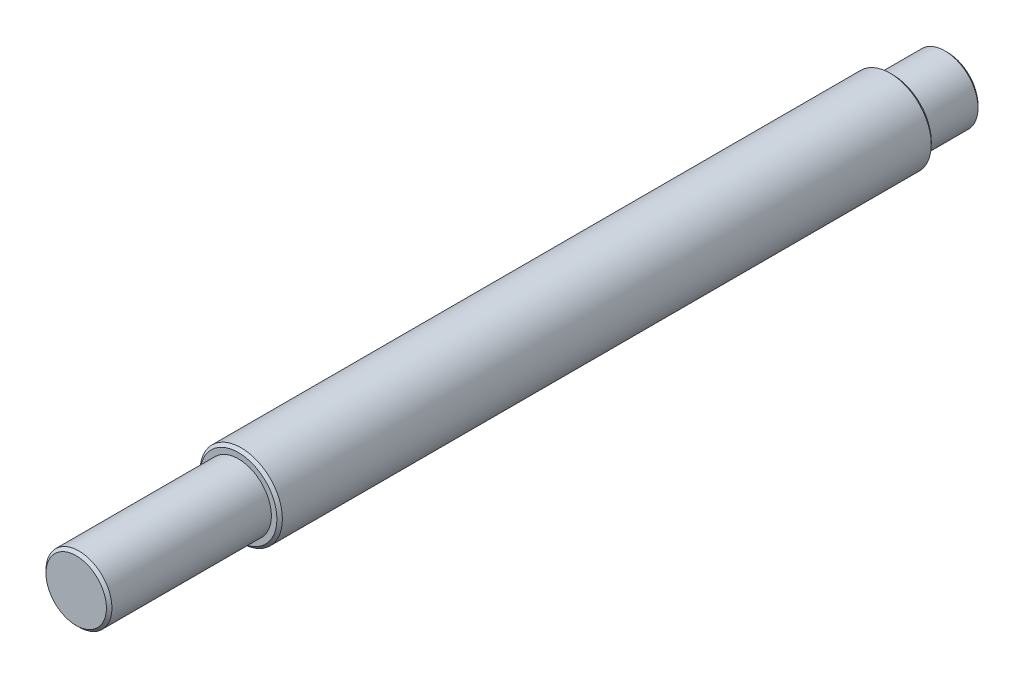
SolidWorks part; units mm, degrees
material "45#"
ref_plane "Front" through (0, 0, 0) normal (0, 0, 1) x (1, 0, 0)
ref_plane "Top" through (0, 0, 0) normal (0, 1, 0) x (1, 0, 0)
ref_plane "Right" through (0, 0, 0) normal (1, 0, 0) x (0, 0, -1)
sketch "草图1" plane through (0, 0, 0) normal (0, 0, 1) x (1, 0, 0)
  circle A0 centre (0, 0) radius 7.5
  dimension "D1" = 15
extrude "凸台-拉伸1" add sketch "草图1" against normal blind 158.5
sketch "草图2" plane through (0, 0, -158.5) normal (0, 0, -1) x (-1, 0, 0)
  circle A0 centre (0, 0) radius 6
  dimension "D1" = 12
ref_plane "基准面2" through (0, 9, 0) normal (0, 1, 0) x (1, 0, 0)
sketch "草图5" plane through (0, 0, 0) normal (0, 0, 1) x (1, 0, 0)
  circle A0 centre (0, 0) radius 6
  dimension "D1" = 12
extrude "切除-拉伸3" cut sketch "草图5" against normal blind 29.5 flip side to cut
chamfer "倒角2" distance 0.5 angle 45 2 edges at (7.5, 0, -29.5) (6, 0, 0)
extrude "切除-拉伸4" cut sketch "草图2" against normal blind 10 flip side to cut
chamfer "倒角3" distance 0.5 angle 45 2 edges at (-7.5, 0, -148.5) (-6, 0, -158.5)
sketch "草图8" plane through (0, 0, 0) normal (0, 1, 0) x (1, 0, 0)
  line L0 (0, 57.5) -> (0, 32.5) construction
  line L1 (2.5, 57.5) -> (2.5, 32.5)
  line L2 (-2.5, 57.5) -> (-2.5, 32.5)
  line L3 (0, 0) -> (0, 32.5) construction
  line L4 (0, 145.5) -> (0, 120.5) construction
  line L5 (2.5, 145.5) -> (2.5, 120.5)
  line L6 (-2.5, 145.5) -> (-2.5, 120.5)
  line L7 (0, 158.5) -> (0, 145.5) construction
  line L8 (5.5, 158.5) -> (-5.5, 158.5) construction
  line L9 (7, 148.5) -> (-7, 148.5) construction
  line L12 (-6, 29.5) -> (6, 29.5) construction
  arc A0 (2.5, 57.5) -> (-2.5, 57.5) centre (0, 57.5) ccw
  arc A1 (-2.5, 32.5) -> (2.5, 32.5) centre (0, 32.5) ccw
  arc A2 (2.5, 145.5) -> (-2.5, 145.5) centre (0, 145.5) ccw
  arc A3 (-2.5, 120.5) -> (2.5, 120.5) centre (0, 120.5) ccw
  point P3 (0, 45)
  point P12 (0, 133)
  dimension "D2" = 3
  dimension "D3" = 25
  dimension "D1" = 5
  dimension "D5" = 3
extrude "切除-拉伸5" cut sketch "草图8" against normal blind 48 from offset 4 offset against normal yes
